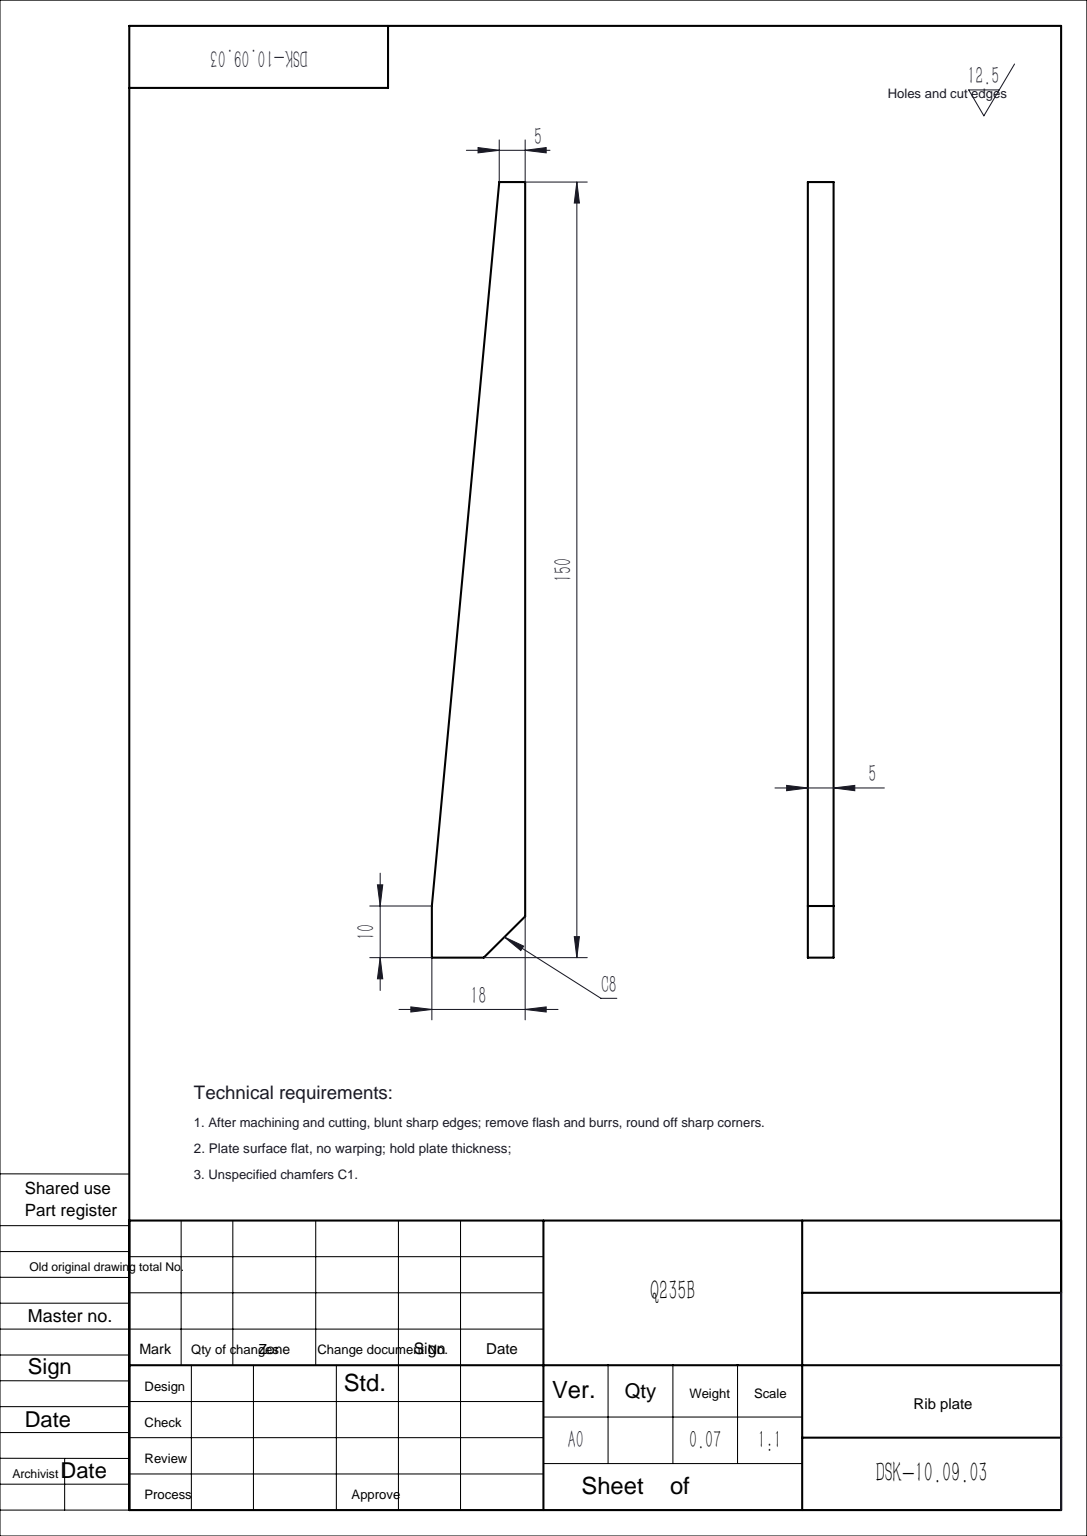
SolidWorks part; units mm, degrees
material "Q235B"
ref_plane "Front Plane" through (0, 0, 0) normal (0, 0, 1) x (1, 0, 0)
ref_plane "Top Plane" through (0, 0, 0) normal (0, 1, 0) x (1, 0, 0)
ref_plane "Right Plane" through (0, 0, 0) normal (1, 0, 0) x (0, 0, -1)
sketch "Sketch1" plane through (0, 0, 0) normal (0, 0, 1) x (1, 0, 0)
  line L0 (0, 0) -> (0, 10)
  line L1 (0, 10) -> (13, 150)
  line L2 (13, 150) -> (18, 150)
  line L3 (18, 150) -> (18, 8)
  line L4 (18, 8) -> (10, 0)
  line L5 (10, 0) -> (0, 0)
  dimension "D1" = 18
  dimension "D2" = 10
  dimension "D3" = 150
  dimension "D4" = 5
  dimension "D5" = 45
  dimension "D6" = 8
extrude "Boss-Extrude1" add sketch "Sketch1" along normal blind 5
